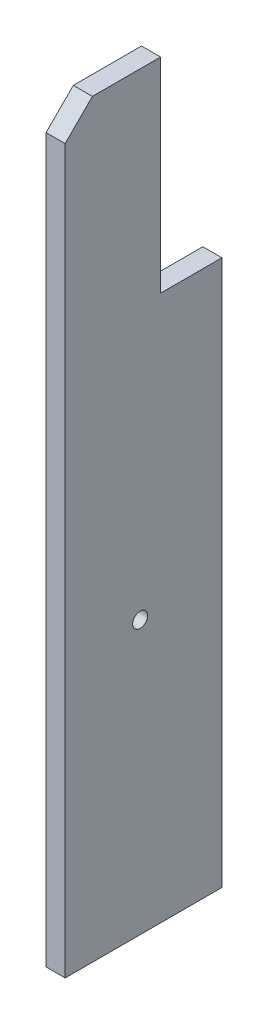
from build123d import *

# Parameters (mm, degrees)
EXTRUDE_1_DEPTH     = 7
CUT_EXTRUDE_2_REACH = 408.32
SKETCH_3_R          = 5.5
CHAMFER_1_SIZE      = 20


with BuildPart() as part:
    # 草图1 → 凸台-拉伸1 (new, symmetric)
    with BuildSketch(Plane(origin=(0, 0, 0), x_dir=(0, 0, -1), z_dir=(1, 0, 0))):
        Polygon((0, 0), (45, 0), (45, -400), (-70, -400), (-70, 150), (0, 150), align=None)
    extrude(amount=EXTRUDE_1_DEPTH, both=True)

    # 草图3 → 切除-拉伸2 (cut, up to next)
    with BuildSketch(Plane(origin=(7, 0, 0), x_dir=(0, 0, -1), z_dir=(1, 0, 0)), mode=Mode.PRIVATE) as cut_extrude_2_sk1:
        with Locations((-15, -200)):
            Circle(SKETCH_3_R)
    cut_extrude_2_tool1 = extrude(cut_extrude_2_sk1.sketch, amount=-CUT_EXTRUDE_2_REACH, mode=Mode.PRIVATE) & part.part
    add(cut_extrude_2_tool1.solids().sort_by_distance((7, -200, 15))[0], mode=Mode.SUBTRACT)

    # 倒角1
    chamfer_1_edges = [part.edges().sort_by_distance(p)[0] for p in [
        (0, 150, 70),
    ]]
    chamfer(chamfer_1_edges, length=CHAMFER_1_SIZE)


solid = part.part
